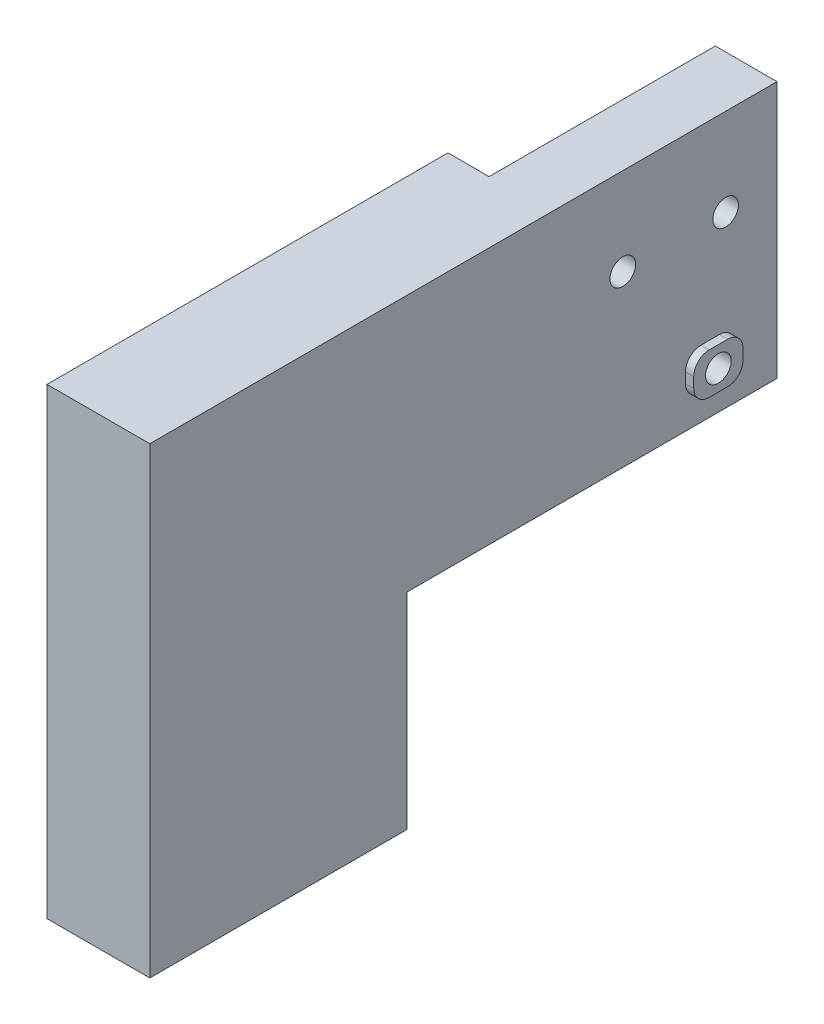
SolidWorks part; units mm, degrees
ref_plane "Front Plane" through (0, 0, 0) normal (0, 0, 1) x (1, 0, 0)
ref_plane "Top Plane" through (0, 0, 0) normal (0, 1, 0) x (1, 0, 0)
ref_plane "Right Plane" through (0, 0, 0) normal (1, 0, 0) x (0, 0, -1)
sketch "Sketch1" plane through (0, 0, 0) normal (0, 0, 1) x (1, 0, 0)
  line L0 (-15, 0) -> (0, 0)
  line L1 (0, 0) -> (0, 45)
  dimension "D1" = 15
  dimension "D2" = 45
extrude "Extrude-Thin1" add sketch "Sketch1" along normal blind 25 thin
sketch "Sketch2" plane through (0, 0, 0) normal (-1, 0, 0) x (0, 0, 1)
  line L1 (0, 45) -> (-36, 45)
  line L2 (0, 45) -> (0, 20)
  line L3 (0, 20) -> (-36, 20)
  line L4 (-36, 45) -> (-36, 20)
  dimension "D1" = 36
  dimension "D2" = 25
extrude "Boss-Extrude1" add sketch "Sketch2" against normal up to surface (10 mm away) up to face at (10, 17.5, 12.5)
sketch "Sketch5" plane through (0, 45, 0) normal (0, 1, 0) x (1, 0, 0)
  line L0 (10, -25) -> (10, 36) construction
  line L1 (0, 36) -> (4, 36)
  line L2 (0, 36) -> (0, 14)
  line L3 (0, 14) -> (4, 14)
  line L4 (4, 36) -> (4, 14)
  dimension "D1" = 6
  dimension "D2" = 22
extrude "Cut-Extrude1" cut sketch "Sketch5" against normal through all
sketch "Sketch6" plane through (0, -10, 0) normal (0, -1, 0) x (1, 0, 0)
  line L1 (-60.0459, 43.3742) -> (33.9268, 43.3742)
  line L2 (-60.0459, 43.3742) -> (-60.0459, -11.0535)
  line L3 (-60.0459, -11.0535) -> (33.9268, -11.0535)
  line L4 (33.9268, 43.3742) -> (33.9268, -11.0535)
extrude "Cut-Extrude2" cut sketch "Sketch6" against normal blind 10
hole_wizard "M5 Tapped Hole1" positions "Sketch7" profile "Sketch8" tap size "M5" standard "ISO"
sketch "Sketch7" plane through (0, 0, 0) normal (0, -1, 0) x (-1, 0, 0)
  line L0 (-10, -12.5) -> (-17.2217, -12.5) construction
  line L1 (-10, 0) -> (-10, -25) construction
  line L3 (-5, -25) -> (-5, -19.5) construction
  line L4 (-10, -25) -> (0, -25) construction
  point P0 (-5, -5.5)
  point P2 (-5, -19.5)
  dimension "D1" = 14
sketch "Sketch8" plane through (5, 0, 5.5) normal (1, 0, 0) x (0, 0, -1)
  line L0 (0, 0) -> (0, 13.6618)
  line L1 (0, 13.6618) -> (2.1, 12.4)
  line L2 (2.1, 12.4) -> (2.1, 0)
  line L5 (2.1, 0) -> (0, 0)
  line L10 (0, 13.6618) -> (-2.1, 12.4) construction
  line L11 (0, -6.35) -> (0, 107.95) construction
  dimension "螺纹孔钻头直径" = 4.2
  dimension "螺纹孔钻头深度" = 12.4
  dimension "导头角度" = 118
cosmetic thread "Cosmetic Thread2" parameters "D1"=10, "D2"=5
cosmetic thread "Cosmetic Thread3" parameters "D1"=10, "D2"=5
hole_wizard "M3 Tapped Hole1" positions "Sketch9" profile "Sketch10" tap size "M3" standard "ISO" end condition through all
sketch "Sketch9" plane through (10, 0, 0) normal (1, 0, 0) x (0, 0, -1)
  line L0 (36, 20) -> (36, 45) construction
  line L1 (-25, 45) -> (36, 45) construction
  point P0 (21, 36.5)
  point P2 (31, 36.5)
  dimension "D1" = 10
  dimension "D2" = 5
  dimension "D3" = 8.5
sketch "Sketch10" plane through (10, 36.5, -21) normal (0, 1, 0) x (0, 0, -1)
  line L0 (0, 0) -> (0, 10)
  line L1 (0, 10) -> (1.25, 10)
  line L2 (1.25, 10) -> (1.25, 0)
  line L5 (1.25, 0) -> (0, 0)
  line L11 (0, -6.35) -> (0, 107.95) construction
  dimension "通孔螺纹孔钻头直径" = 2.5
  dimension "通孔螺纹孔钻头深度" = 10
cosmetic thread "Cosmetic Thread4" parameters "D2"=3
cosmetic thread "Cosmetic Thread5" parameters "D2"=3
sketch "Sketch12" plane through (10, 0, 0) normal (1, 0, 0) x (0, 0, -1)
  line L0 (36, 20) -> (36, 45) construction
  line L1 (27.1, 26.5) -> (31.9, 26.5)
  line L2 (27.1, 26.5) -> (27.1, 22.5)
  line L3 (27.1, 22.5) -> (31.9, 22.5)
  line L4 (31.9, 26.5) -> (31.9, 22.5)
  line L5 (27.1, 26.5) -> (31.9, 22.5) construction
  line L6 (27.1, 22.5) -> (31.9, 26.5) construction
  line L7 (0, 20) -> (36, 20) construction
  point P0 (29.5, 24.5)
  dimension "D1" = 6.5
  dimension "D2" = 4.5
  dimension "D3" = 4.8
  dimension "D4" = 4
extrude "Boss-Extrude2" add sketch "Sketch12" along normal blind 0.8
hole_wizard "M3 Tapped Hole2" positions "Sketch3" profile "Sketch4" tap size "M3" standard "ISO" end condition through all
sketch "Sketch3" plane through (0, 0, 0) normal (-1, 0, 0) x (0, 0, 1)
  line L2 (-36, 45) -> (-36, 20) construction
  line L3 (-14, 20) -> (0, 20) construction
  point P0 (-29.5, 24.5)
  dimension "D1" = 6.5
  dimension "D2" = 4.5
sketch "Sketch4" plane through (0, 24.5, -29.5) normal (0, 1, 0) x (0, 0, 1)
  line L0 (0, 0) -> (0, 10.8)
  line L1 (0, 10.8) -> (1.25, 10.8)
  line L2 (1.25, 10.8) -> (1.25, 0)
  line L5 (1.25, 0) -> (0, 0)
  line L11 (0, -6.35) -> (0, 107.95) construction
  dimension "通孔螺纹孔钻头直径" = 2.5
  dimension "通孔螺纹孔钻头深度" = 10.8
cosmetic thread "Cosmetic Thread1" parameters "D2"=3
fillet "Fillet1" radius 1.5 4 edges at (10.4, 22.5, -27.1) (10.4, 22.5, -31.9) (10.4, 26.5, -31.9) (10.4, 26.5, -27.1)
